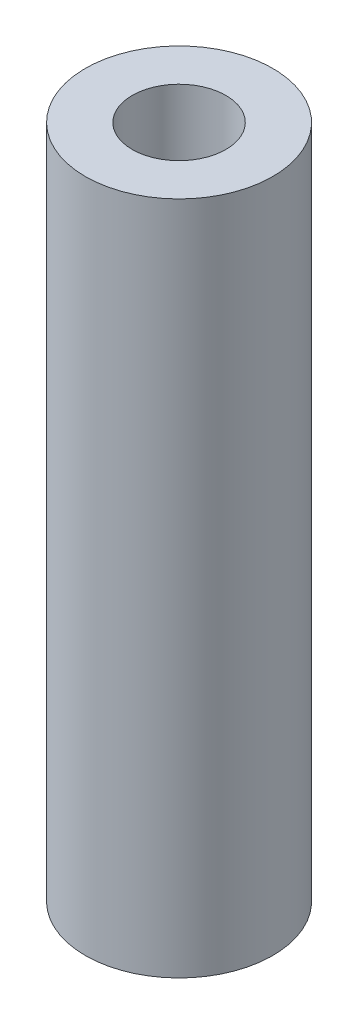
SolidWorks part; units mm, degrees
material "6061 合金"
ref_plane "前视基准面" through (0, 0, 0) normal (0, 0, 1) x (1, 0, 0)
ref_plane "上视基准面" through (0, 0, 0) normal (0, 1, 0) x (1, 0, 0)
ref_plane "右视基准面" through (0, 0, 0) normal (1, 0, 0) x (0, 0, -1)
sketch "草图1" plane through (0, 0, 0) normal (0, 1, 0) x (1, 0, 0)
  circle A0 centre (0, 0) radius 2.5
  dimension "D1" = 5
extrude "凸台-拉伸1" add sketch "草图1" along normal blind 18
sketch "草图2" plane through (0, 18, 0) normal (0, 1, 0) x (1, 0, 0)
  point P0 (0, 0)
hole_wizard "M3 螺纹孔1" positions "草图2" profile "草图3" tap size "M3" standard "GB" end condition through all
sketch "草图3" plane through (0, 18, 0) normal (1, 0, 0) x (0, 0, 1)
  line L0 (0, 0) -> (0, 18)
  line L1 (0, 18) -> (1.25, 18)
  line L2 (1.25, 18) -> (1.25, 0)
  line L5 (1.25, 0) -> (0, 0)
  line L11 (0, -6.35) -> (0, 107.95) construction
  dimension "通孔螺纹孔钻头直径" = 2.5
  dimension "通孔螺纹孔钻头深度" = 18
cosmetic thread "孔螺纹线1" parameters "D2"=3
